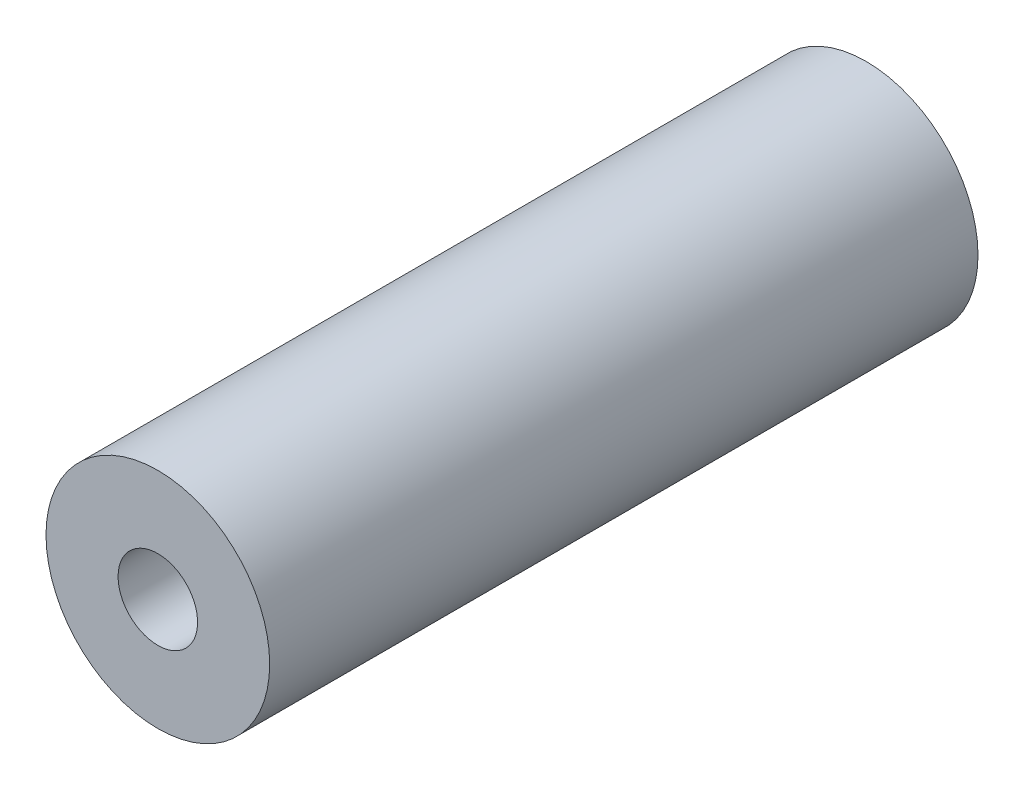
SolidWorks part; units mm, degrees
ref_plane "前视基准面" through (0, 0, 0) normal (0, 0, 1) x (1, 0, 0)
ref_plane "上视基准面" through (0, 0, 0) normal (0, 1, 0) x (1, 0, 0)
ref_plane "右视基准面" through (0, 0, 0) normal (1, 0, 0) x (0, 0, -1)
sketch "草图1" plane through (0, 0, 0) normal (0, 0, 1) x (1, 0, 0)
  circle A0 centre (0, 0) radius 1.6
  circle A1 centre (0, 0) radius 4.5
  dimension "D1" = 3.2
  dimension "D2" = 9
extrude "凸台-拉伸1" add sketch "草图1" along normal mid plane 28.5
